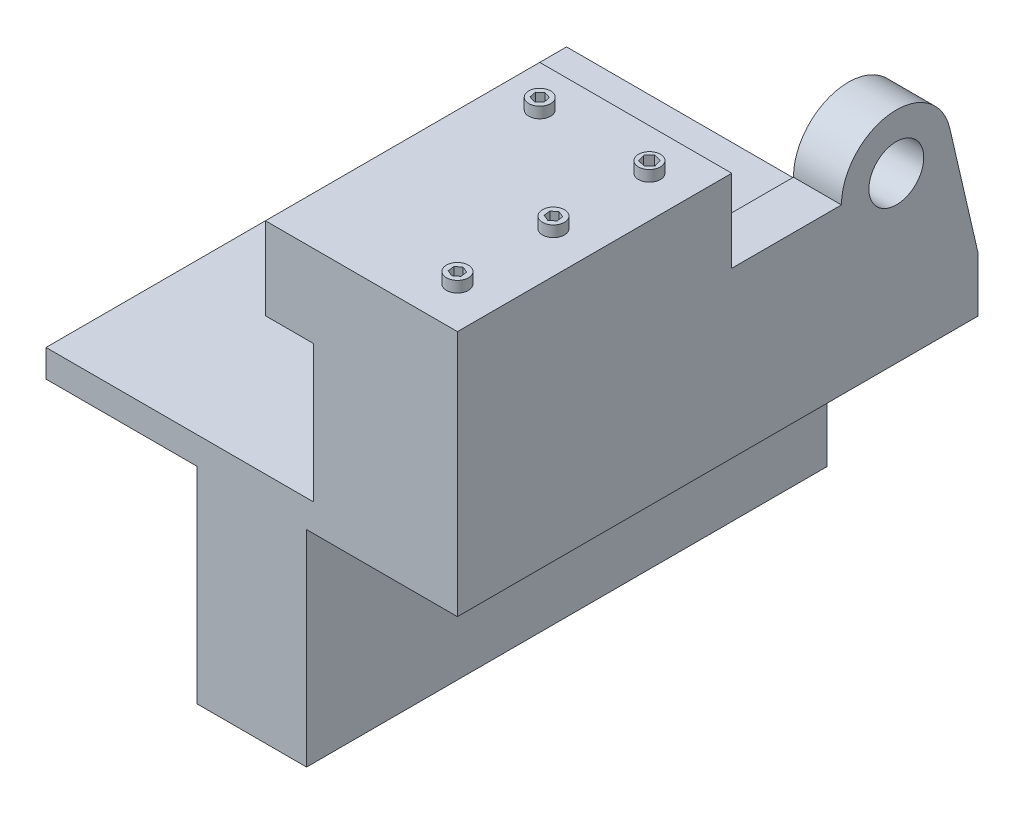
from build123d import *

# Parameters (mm, degrees)
SKETCH1_W           = 70
SKETCH1_H           = 100
BOSS_EXTRUDE1_DEPTH = 30
SKETCH2_R           = 4
BOSS_EXTRUDE2_DEPTH = 4
SKETCH3_W           = 35
SKETCH3_H           = 100
BOSS_EXTRUDE3_DEPTH = 40
SKETCH4_R           = 10
BOSS_EXTRUDE4_DEPTH = 17.5
BOSS_EXTRUDE5_DEPTH = 10
SKETCH6_W           = 150
SKETCH6_H           = 189.781220368
BOSS_EXTRUDE6_DEPTH = 10
SKETCH7_W           = 40
SKETCH7_H           = 189.781220368
BOSS_EXTRUDE7_DEPTH = 75
SKETCH8_W           = 213.425004002
SKETCH8_H           = 201.568059336
CUT_EXTRUDE1_DEPTH  = 210


with BuildPart() as part:
    # Sketch1 → Boss-Extrude1 (new body)
    with BuildSketch(Plane(origin=(0, 0, 0), x_dir=(1, 0, 0), z_dir=(0, 1, 0))):
        Rectangle(SKETCH1_W, SKETCH1_H)
    extrude(amount=BOSS_EXTRUDE1_DEPTH)

    # Sketch2 → Boss-Extrude2 (add)
    # profile 1 of 4: a face of its own
    with BuildSketch(Plane(origin=(0, 30, 0), x_dir=(1, 0, 0), z_dir=(0, 1, 0))):
        with Locations(Location((-20, -35, 0), (0, 0, 270))):
            Circle(SKETCH2_R)
        Polygon((-18.132531053, -36.656757487), (-17.631471454, -34.211103194), (-19.498940402, -32.554345707), (-21.867468947, -33.343242513), (-22.368528546, -35.788896806), (-20.501059598, -37.445654293), align=None, mode=Mode.SUBTRACT)
    # profile 2 of 4: a face of its own
    with BuildSketch(Plane(origin=(0, 30, 0), x_dir=(1, 0, 0), z_dir=(0, 1, 0))):
        with Locations(Location((20, -35, 0), (0, 0, 270))):
            Circle(SKETCH2_R)
        Polygon((21.913058762, -37.035169602), (22.719037957, -34.360827314), (20.805979195, -32.325657712), (18.086941238, -32.964830398), (17.280962043, -35.639172686), (19.194020805, -37.674342288), align=None, mode=Mode.SUBTRACT)
    # profile 3 of 4: a face of its own
    with BuildSketch(Plane(origin=(0, 30, 0), x_dir=(1, 0, 0), z_dir=(0, 1, 0))):
        with Locations(Location((20, 0, 0), (0, 0, 270))):
            Circle(SKETCH2_R)
        Polygon((21.913058762, -1.47020522), (22.229764451, 0.921654877), (20.316705689, 2.391860097), (18.086941238, 1.47020522), (17.770235549, -0.921654877), (19.683294311, -2.391860097), align=None, mode=Mode.SUBTRACT)
    # profile 4 of 4: a face of its own
    with BuildSketch(Plane(origin=(0, 30, 0), x_dir=(1, 0, 0), z_dir=(0, 1, 0))):
        with Locations(Location((20, 35, 0), (0, 0, 270))):
            Circle(SKETCH2_R)
        Polygon((21.913058762, 33.534680981), (22.225532876, 35.924097978), (20.312474114, 37.389416996), (18.086941238, 36.465319019), (17.774467124, 34.075902022), (19.687525886, 32.610583004), align=None, mode=Mode.SUBTRACT)
    extrude(amount=BOSS_EXTRUDE2_DEPTH)

    # Sketch3 → Boss-Extrude3 (add)
    with BuildSketch(Plane.XZ):
        Rectangle(SKETCH3_W, SKETCH3_H)
    extrude(amount=BOSS_EXTRUDE3_DEPTH)

    # Sketch4 → Boss-Extrude4 (add)
    with BuildSketch(Plane(origin=(17.5, 0, 0), x_dir=(0, 0, -1), z_dir=(1, 0, 0))):
        with BuildLine():
            Line((-50, -40), (-139.781220368, -40))
            Line((-139.781220368, -40), (-129.48544067, 4.507505064))
            ThreePointArc((-129.48544067, 4.507505064), (-107.731609976, 19.87094378), (-90, 0))
            Line((-90, 0), (-50, 0))
            Line((-50, 0), (50, 0))
            Line((50, 0), (50, -40))
            Line((50, -40), (-50, -40))
        make_face()
        with Locations(Location((-110, 0, 0), (0, 0, 180))):
            Circle(SKETCH4_R, mode=Mode.SUBTRACT)
    extrude(amount=BOSS_EXTRUDE4_DEPTH)

    # Sketch5 → Boss-Extrude5 (add)
    with BuildSketch(Plane.XZ.offset(40)):
        Polygon((17.5, 139.781220368), (35, 139.781220368), (35, -50), (-17.5, -50), (-17.5, 50), (17.5, 50), align=None)
    extrude(amount=BOSS_EXTRUDE5_DEPTH)

    # Sketch6 → Boss-Extrude6 (add)
    with BuildSketch(Plane.XZ.offset(50)):
        with Locations((-40, 44.890610184)):
            Rectangle(SKETCH6_W, SKETCH6_H)
    extrude(amount=BOSS_EXTRUDE6_DEPTH)

    # Sketch7 → Boss-Extrude7 (add)
    with BuildSketch(Plane.XZ.offset(60)):
        with Locations((-40, 44.890610184)):
            Rectangle(SKETCH7_W, SKETCH7_H)
    extrude(amount=BOSS_EXTRUDE7_DEPTH)

    # Mirror3: part across plane


with BuildPart() as part_1:
    add(part.part)
    add(part.part.mirror(Plane(origin=(17.5, -50, 139.781220368), x_dir=(1, 0, 0), z_dir=(0, 0, -1))))

    # Sketch8 → Cut-Extrude1 (cut)
    with BuildSketch(Plane.XY.offset(139.781220368)):
        with Locations((-37.145550358, -46.351954617)):
            Rectangle(SKETCH8_W, SKETCH8_H)
    extrude(amount=-CUT_EXTRUDE1_DEPTH, mode=Mode.SUBTRACT)


solid = part_1.part
